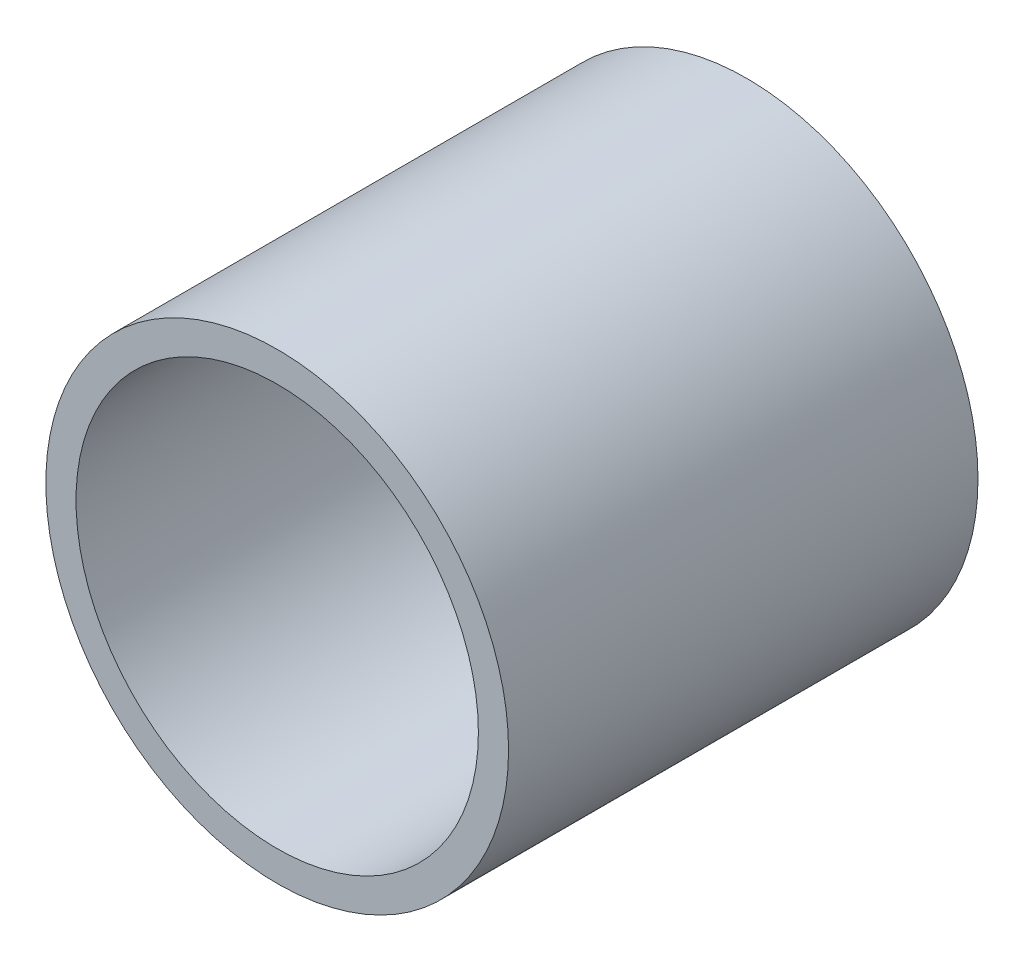
from build123d import *

# Parameters (mm, degrees)
SKETCH1_R           = 3.45
SKETCH1_R_2         = 3
BOSS_EXTRUDE1_DEPTH = 7


with BuildPart() as part:
    # Sketch1 → Boss-Extrude1 (new body)
    with BuildSketch(Plane.XY):
        Circle(SKETCH1_R)
        Circle(SKETCH1_R_2, mode=Mode.SUBTRACT)
    extrude(amount=BOSS_EXTRUDE1_DEPTH)


solid = part.part
